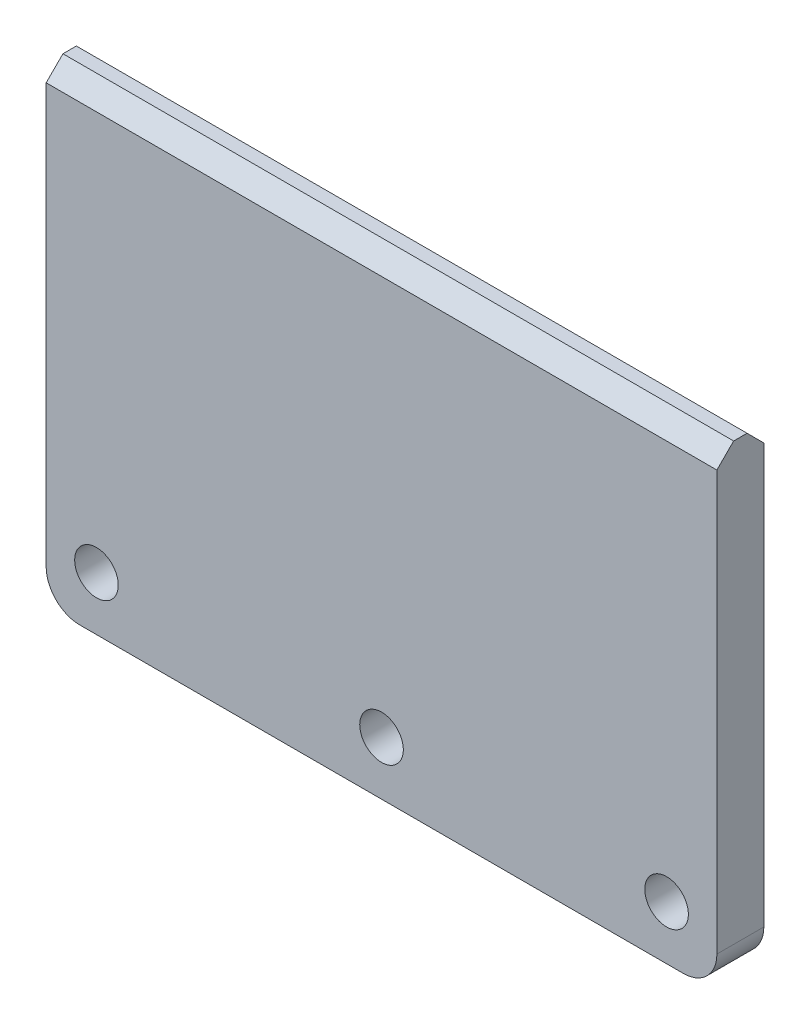
from build123d import *

# Parameters (mm, degrees)
SKETCH1_W           = 200
SKETCH1_H           = 140
BOSS_EXTRUDE1_DEPTH = 14
CHAMFER1_SIZE       = 5
SKETCH3_R           = 6.5
CUT_EXTRUDE2_DEPTH  = 245.532206468
FILLET1_R           = 10


with BuildPart() as part:
    # Sketch1 → Boss-Extrude1 (new body)
    with BuildSketch(Plane.XY):
        with Locations((100, 70)):
            Rectangle(SKETCH1_W, SKETCH1_H)
    extrude(amount=BOSS_EXTRUDE1_DEPTH)

    # Chamfer1
    chamfer1_edges = [part.edges().sort_by_distance(p)[0] for p in [
        (100, 140, 14),
        (100, 140, 0),
    ]]
    chamfer(chamfer1_edges, length=CHAMFER1_SIZE)

    # Sketch3 → Cut-Extrude2 (cut, through all)
    with BuildSketch(Plane(origin=(0, 0, 0), x_dir=(-1, 0, 0), z_dir=(0, 0, -1))):
        with Locations((-185, 16)):
            Circle(SKETCH3_R)
        with Locations((-100, 16)):
            Circle(SKETCH3_R)
        with Locations((-15, 16)):
            Circle(SKETCH3_R)
    extrude(amount=-CUT_EXTRUDE2_DEPTH, mode=Mode.SUBTRACT)

    # Fillet1
    fillet1_edges = [part.edges().sort_by_distance(p)[0] for p in [
        (200, 0, 7),
        (0, 0, 7),
    ]]
    fillet(fillet1_edges, radius=FILLET1_R)


solid = part.part
